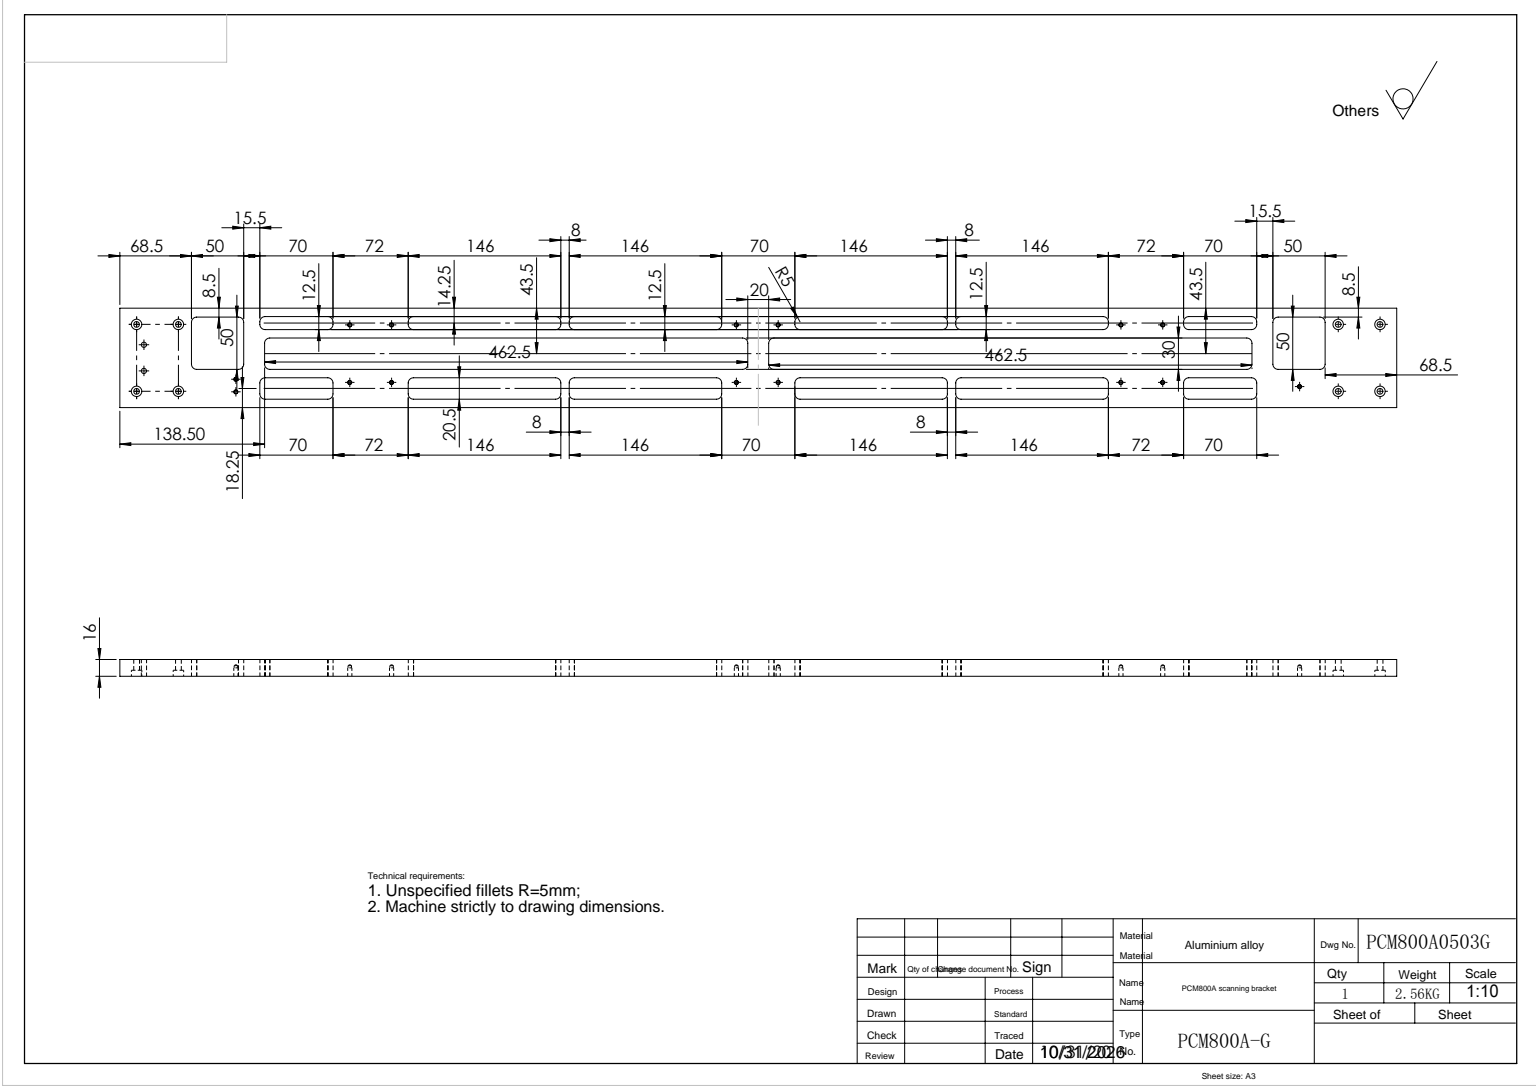
SolidWorks part; units mm, degrees
ref_plane "前视" through (0, 0, 0) normal (0, 0, 1) x (1, 0, 0)
ref_plane "上视" through (0, 0, 0) normal (0, 1, 0) x (1, 0, 0)
ref_plane "右视" through (0, 0, 0) normal (1, 0, 0) x (0, 0, -1)
sketch "草图1" plane through (0, 0, 0) normal (0, 0, 1) x (1, 0, 0)
  line L1 (0, 0) -> (95, 0)
  line L2 (0, 0) -> (0, 16)
  line L3 (0, 16) -> (95, 16)
  line L4 (95, 0) -> (95, 16)
  dimension "D1" = 16
  dimension "D2" = 95
extrude "拉伸1" add sketch "草图1" along normal blind 1222
hole_wizard "打孔尺寸根据内六角圆柱头螺钉的类型1" positions "3D草图1" profile "草图4" counterbore size "M5" standard "GB" end condition through all
sketch3d "3D草图1"
  line L0 (0, 16, 1222) -> (0, 16, 0) construction
  line L1 (95, 16, 0) -> (0, 16, 0) construction
  point P0 (15.5, 16, 16)
  dimension "D1" = 15.5
  dimension "D2" = 16
sketch "草图4" plane through (15.5, 16, 16) normal (1, 0, 0) x (0, 0, 1)
  line L0 (0, 0) -> (0, 16)
  line L1 (0, 16) -> (2.75, 16)
  line L3 (2.75, 16) -> (2.75, 5.7)
  line L4 (2.75, 5.7) -> (5, 5.7)
  line L5 (5, 5.7) -> (5, 0)
  line L7 (5, 0) -> (0, 0)
  line L11 (0, -6.35) -> (0, 107.95) construction
  dimension "籵謂謂眻噤" = 5.5
  dimension "籵謂謂旮僅" = 16
  dimension "翐倛麥芛謂眻噤" = 10
  dimension "翐倛麥芛謂旮僅" = 5.7
pattern_linear "阵列(线性)1" count 2 spacing 40 along (0, 0, 1) count 2 spacing 64 along (1, 0, 0) of "打孔尺寸根据内六角圆柱头螺钉的类型1"
hole_wizard "M5 螺纹孔1" positions "3D草图2" profile "草图16" tap size "M5" standard "GB" end condition through all
sketch3d "3D草图2"
  line L0 (95, 16, 0) -> (0, 16, 0) construction
  line L1 (95, 16, 1222) -> (95, 16, 0) construction
  point P0 (35, 16, 23)
  point P2 (60, 16, 23)
  dimension "D1" = 25
  dimension "D2" = 23
  dimension "D3" = 23
  dimension "D4" = 35
sketch "草图16" plane through (35, 16, 23) normal (1, 0, 0) x (0, 0, 1)
  line L0 (0, 0) -> (0, 16)
  line L1 (0, 16) -> (2.5, 16)
  line L2 (2.5, 16) -> (2.5, 0)
  line L5 (2.5, 0) -> (0, 0)
  line L11 (0, -6.35) -> (0, 107.95) construction
  dimension "螺纹线主直径" = 5
  dimension "通孔螺纹孔钻头深度" = 16
pattern_linear "阵列(线性)18" count 2 spacing 1150 along (0, 0, 1) of "打孔尺寸根据内六角圆柱头螺钉的类型1", "阵列(线性)1"
hole_wizard "M4 螺纹孔1" positions "草图18" profile "草图17" tap size "M4" standard "GB"
sketch "草图18" plane through (0, 16, 0) normal (0, 1, 0) x (-1, 0, 0)
  line L0 (-79, 0) -> (-79, 1222) construction
  line L1 (-95, 0) -> (0, 0) construction
  line L2 (-95, 1222) -> (0, 1222) construction
  line L4 (-24, 0) -> (-24, 1222) construction
  line L6 (-95, 1222) -> (-95, 0) construction
  line L7 (0, 1222) -> (0, 0) construction
  point P0 (-79, 260)
  point P1 (-79, 220)
  point P3 (-24, 220)
  point P5 (-24, 260)
  point P7 (-79, 630)
  point P9 (-24, 590)
  point P11 (-79, 590)
  point P13 (-24, 630)
  point P15 (-79, 958)
  point P17 (-24, 958)
  point P19 (-79, 998)
  point P21 (-24, 998)
  point P23 (-20, 1129)
  point P25 (-27, 111)
  point P27 (-15, 111)
  dimension "D1" = 260
  dimension "D2" = 220
  dimension "D3" = 260
  dimension "D4" = 220
  dimension "D5" = 370
  dimension "D6" = 370
  dimension "D7" = 330
  dimension "D8" = 330
  dimension "D9" = 368
  dimension "D10" = 368
  dimension "D11" = 40
  dimension "D12" = 40
  dimension "D13" = 16
  dimension "D14" = 55
  dimension "D15" = 111
  dimension "D16" = 111
  dimension "D17" = 15
  dimension "D18" = 12
  dimension "D19" = 20
  dimension "D20" = 93
sketch "草图17" plane through (79, 16, 260) normal (1, 0, 0) x (0, 0, 1)
  line L0 (0, 0) -> (0, 11.0914)
  line L1 (0, 11.0914) -> (1.65, 10.1)
  line L2 (1.65, 10.1) -> (1.65, 8)
  line L3 (1.65, 8) -> (2, 8)
  line L4 (2, 8) -> (2, 0)
  line L5 (2, 0) -> (0, 0)
  line L10 (0, 11.0914) -> (-1.65, 10.1) construction
  line L11 (0, -6.35) -> (0, 107.95) construction
  dimension "螺纹孔钻头直径" = 3.3
  dimension "螺纹孔钻头深度" = 10.1
  dimension "螺纹主直径" = 4
  dimension "螺纹深度" = 8
  dimension "导头角度" = 118
sketch "草图20" plane through (0, 16, 0) normal (0, 1, 0) x (1, 0, 0)
  line L0 (51.5, -138.5) -> (51.5, -1083.2439) construction
  line L1 (66.5, -138.5) -> (36.5, -138.5)
  line L2 (66.5, -138.5) -> (66.5, -601)
  line L3 (66.5, -1083.5) -> (36.5, -1083.5)
  line L4 (36.5, -138.5) -> (36.5, -601)
  line L5 (95, 0) -> (0, 0) construction
  line L6 (36.5, -1153.5) -> (86.5, -1153.5)
  line L7 (36.5, -118.5) -> (86.5, -118.5)
  line L8 (36.5, -118.5) -> (36.5, -68.5)
  line L9 (36.5, -68.5) -> (86.5, -68.5)
  line L10 (86.5, -118.5) -> (86.5, -68.5)
  line L11 (0, -611) -> (371.3148, -611) construction
  line L12 (0, -1222) -> (0, 0) construction
  line L13 (36.5, -601) -> (66.5, -601)
  line L14 (36.5, -621) -> (66.5, -621)
  line L15 (66.5, -621) -> (66.5, -1083.5)
  line L16 (36.5, -621) -> (36.5, -1083.5)
  line L17 (8, -426) -> (36.5, -426) construction
  line L18 (8, -276) -> (28.5, -276)
  line L19 (8, -276) -> (8, -422)
  line L20 (8, -576) -> (28.5, -576)
  line L21 (28.5, -276) -> (28.5, -422)
  line L22 (8, -422) -> (28.5, -422)
  line L23 (8, -430) -> (28.5, -430)
  line L24 (28.5, -430) -> (28.5, -576)
  line L25 (8, -430) -> (8, -576)
  line L26 (95, -1222) -> (95, 0) construction
  line L27 (8, -134) -> (28.5, -134)
  line L28 (8, -134) -> (8, -204)
  line L29 (8, -204) -> (28.5, -204)
  line L30 (28.5, -134) -> (28.5, -204)
  line L31 (74.5, -134) -> (87, -134)
  line L32 (74.5, -134) -> (74.5, -204)
  line L33 (74.5, -204) -> (87, -204)
  line L34 (87, -134) -> (87, -204)
  line L35 (74.5, -422) -> (87, -422)
  line L36 (74.5, -276) -> (87, -276)
  line L37 (74.5, -276) -> (74.5, -422)
  line L38 (74.5, -576) -> (87, -576)
  line L39 (87, -276) -> (87, -422)
  line L40 (74.5, -430) -> (87, -430)
  line L41 (74.5, -430) -> (74.5, -576)
  line L42 (87, -430) -> (87, -576)
  line L43 (86.5, -1103.5) -> (86.5, -1153.5)
  line L44 (36.5, -1103.5) -> (36.5, -1153.5)
  line L45 (36.5, -1103.5) -> (86.5, -1103.5)
  line L46 (74.5, -1088) -> (87, -1088)
  line L47 (8, -1088) -> (28.5, -1088)
  line L48 (28.5, -1088) -> (28.5, -1018)
  line L49 (8, -1088) -> (8, -1018)
  line L50 (8, -1018) -> (28.5, -1018)
  line L51 (74.5, -1088) -> (74.5, -1018)
  line L52 (87, -1088) -> (87, -1018)
  line L53 (74.5, -1018) -> (87, -1018)
  line L54 (74.5, -946) -> (87, -946)
  line L55 (8, -946) -> (28.5, -946)
  line L56 (28.5, -792) -> (28.5, -646)
  line L57 (8, -646) -> (28.5, -646)
  line L58 (74.5, -646) -> (87, -646)
  line L59 (8, -792) -> (8, -646)
  line L60 (8, -792) -> (28.5, -792)
  line L61 (87, -946) -> (87, -800)
  line L62 (74.5, -946) -> (74.5, -800)
  line L63 (87, -792) -> (87, -646)
  line L64 (74.5, -792) -> (74.5, -646)
  line L65 (74.5, -792) -> (87, -792)
  line L66 (74.5, -800) -> (87, -800)
  line L67 (8, -946) -> (8, -800)
  line L68 (8, -800) -> (28.5, -800)
  line L69 (28.5, -946) -> (28.5, -800)
  circle A2 centre (79, -220) radius 1.65 construction
  circle A4 centre (24, -958) radius 2 construction
  dimension "D3" = 27.5
  dimension "D1" = 30
  dimension "D2" = 945
  dimension "D4" = 138.5
  dimension "D5" = 20
  dimension "D6" = 50
  dimension "D7" = 50
  dimension "D8" = 10
  dimension "D9" = 20
  dimension "D10" = 8
  dimension "D11" = 8
  dimension "D12" = 35
  dimension "D13" = 300
  dimension "D14" = 4
  dimension "D15" = 4
  dimension "D16" = 185
  dimension "D17" = 72
  dimension "D18" = 70
  dimension "D19" = 8
  dimension "D20" = 8
extrude "切除-拉伸1" cut sketch "草图20" against normal blind 158
fillet "圆角1" radius 5 64 edges at (86.5, 8, 68.5) (86.5, 8, 1103.5) (86.5, 8, 1153.5) (36.5, 8, 1153.5) (36.5, 8, 1103.5) (28.5, 8, 1018) (8, 8, 1018) (28.5, 8, 1088) (8, 8, 1088) (36.5, 8, 1083.5) (66.5, 8, 1083.5) (87, 8, 1088) (74.5, 8, 1088) (87, 8, 1018) (74.5, 8, 1018) (87, 8, 946) (74.5, 8, 946) (28.5, 8, 946) (8, 8, 946) (87, 8, 800) (74.5, 8, 800) (87, 8, 792) (74.5, 8, 792) (28.5, 8, 800) (8, 8, 800) (28.5, 8, 792) (8, 8, 792) (87, 8, 646) (74.5, 8, 646) (8, 8, 646) (28.5, 8, 646) (66.5, 8, 621) (36.5, 8, 621) (87, 8, 576) (74.5, 8, 576) (66.5, 8, 601) (36.5, 8, 601) (28.5, 8, 576) (8, 8, 576) (8, 8, 430) (28.5, 8, 430) (87, 8, 430) (74.5, 8, 430) (87, 8, 422) (74.5, 8, 422) (28.5, 8, 422) (8, 8, 422) (8, 8, 276) (28.5, 8, 276) (87, 8, 276) (74.5, 8, 276) (28.5, 8, 204) (8, 8, 204) (74.5, 8, 204) (87, 8, 204) (8, 8, 134) (28.5, 8, 134) (36.5, 8, 138.5) (66.5, 8, 138.5) (74.5, 8, 134) (87, 8, 134) (36.5, 8, 118.5) (86.5, 8, 118.5) (36.5, 8, 68.5)
